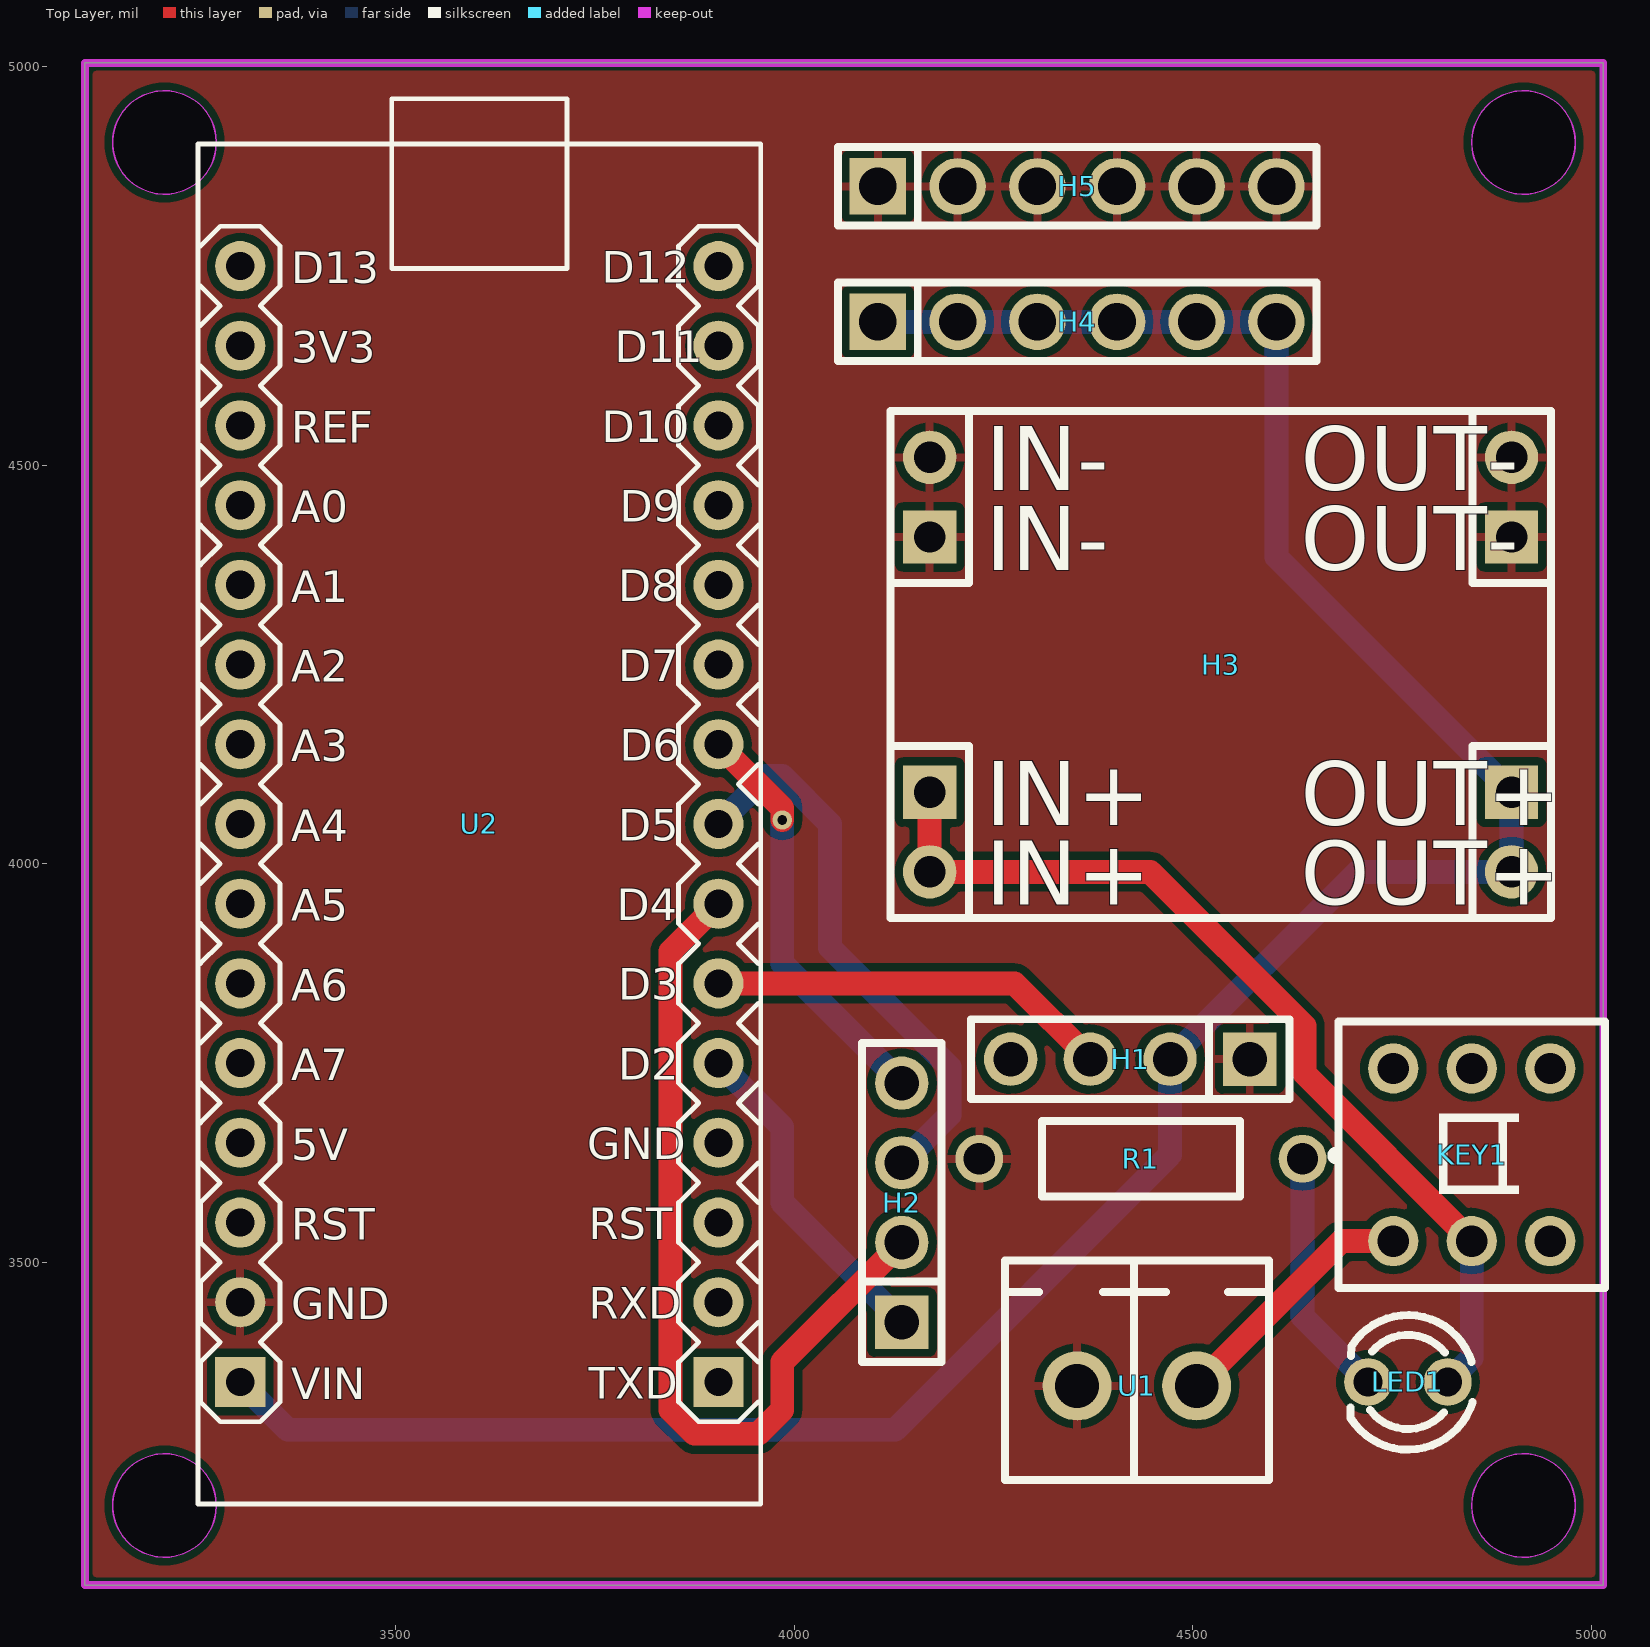
[diagram p0: Top Layer view]
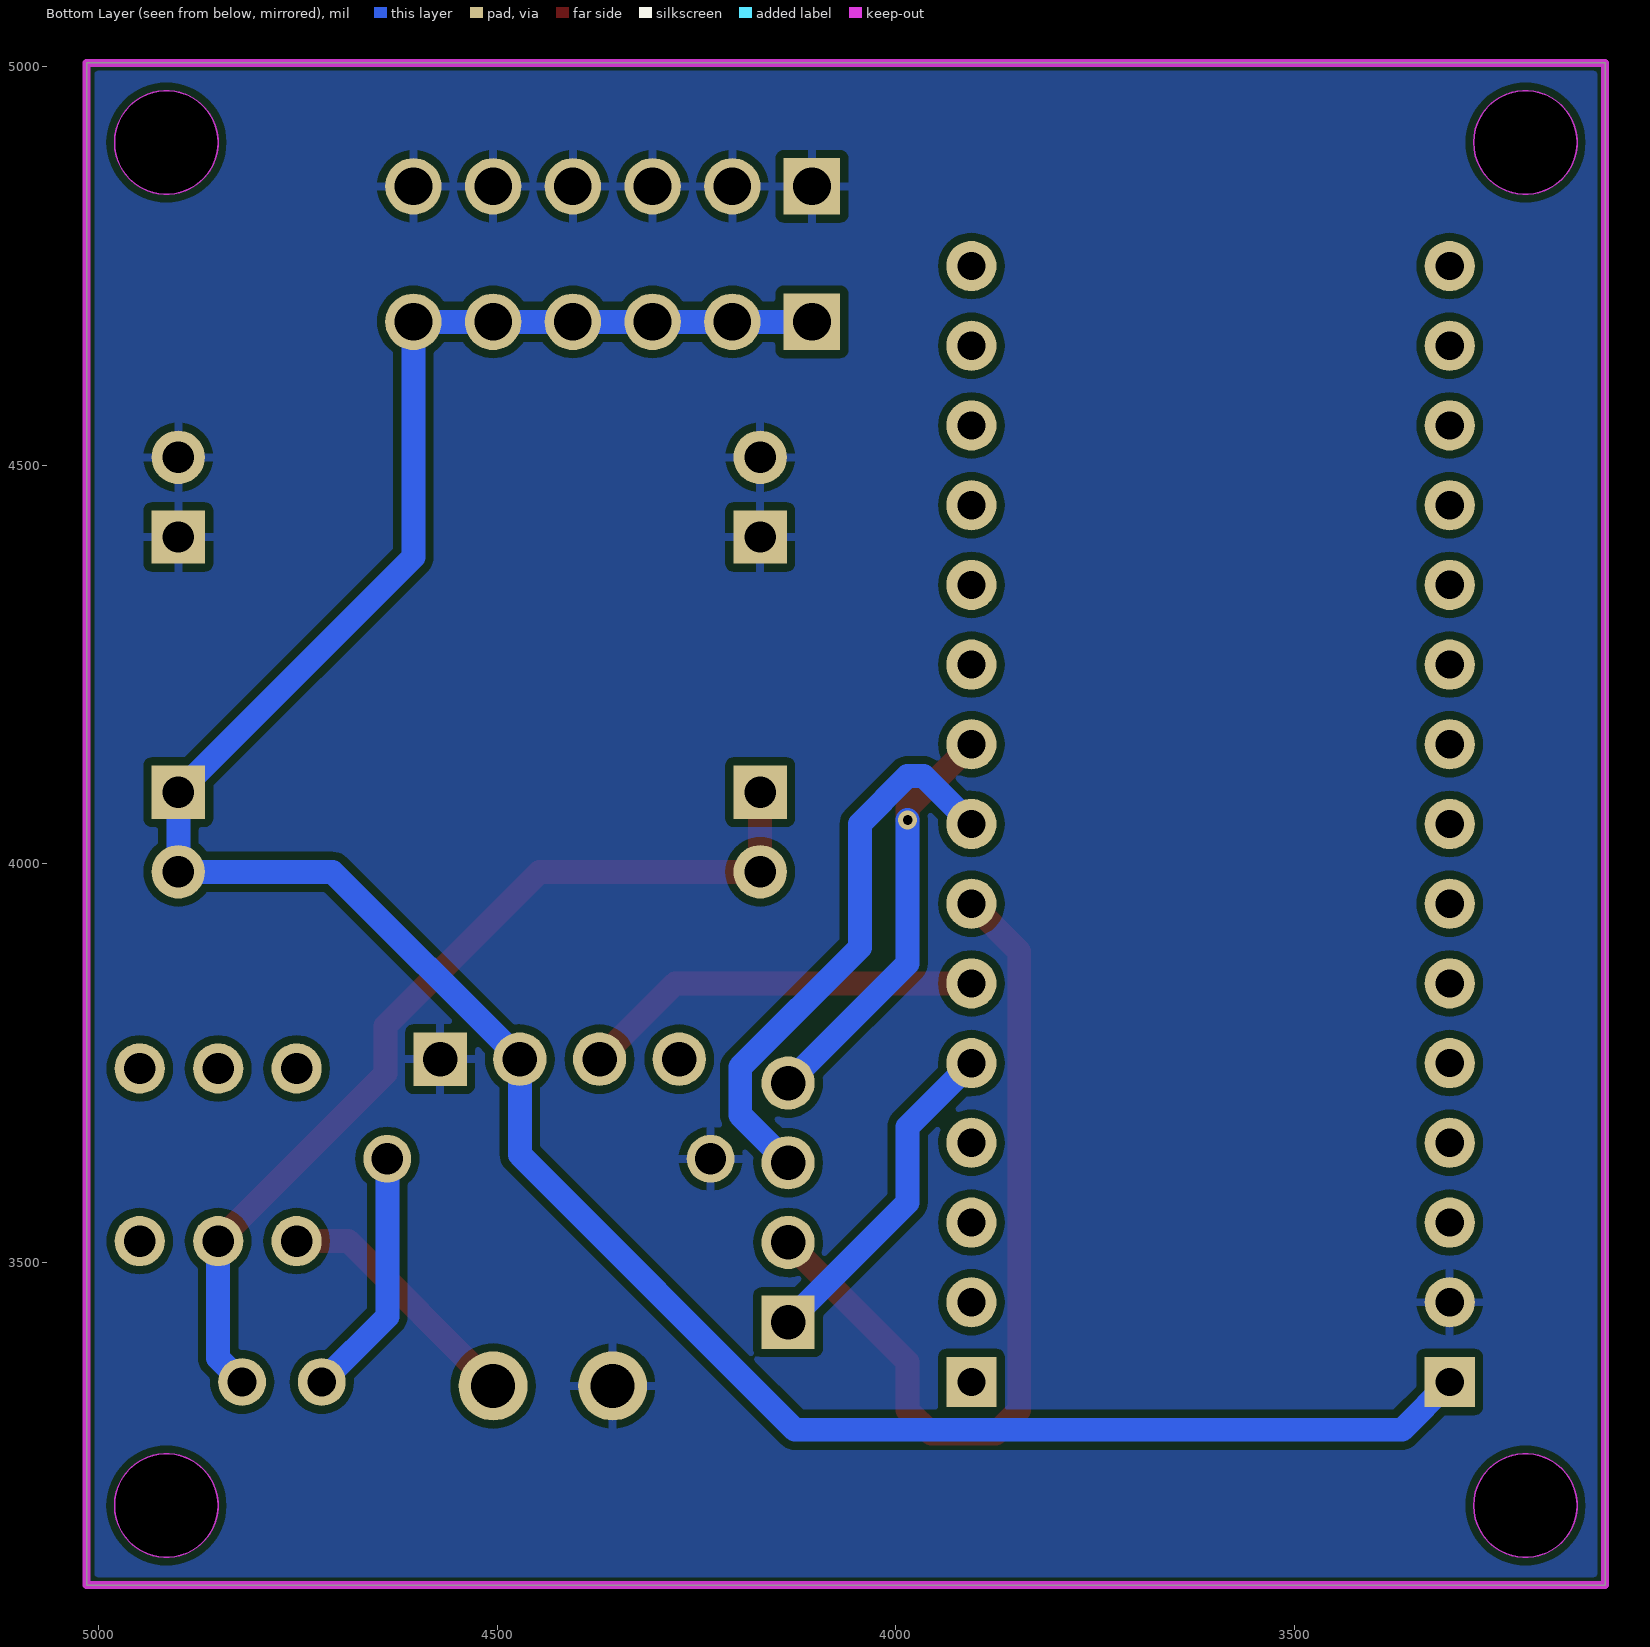
[diagram p1: Bottom Layer view, seen from below]
# Altium PCB MISC49855.pcbdoc
Units mil, origin at the board's own origin, x right, y up, seen from the top; angles counter-clockwise.
Board outline 1905 x 1910 mil, 2 copper layers (Top Layer, Bottom Layer), stack 62.206 mil thick; 10 components, 10 nets, 70 pads, 1 vias.

## Layer stack, top to bottom
Top Solder Mask Layer: solder mask 0.394, Dk 3.3
Top Layer: signal copper 1.379
Dielectric1: surface 59.449, FR4, Dk 4.5
Bottom Layer: signal copper 1.378
Bottom Solder Mask Layer: solder mask 0.394, Dk 3.3

## Board outline
3110,5005 3110,3095 5015,3095 5015,5005
cut-out: 3275,3195 cw(c3210,3195) 3145,3195 cw(c3210,3195)
cut-out: 4980,3195 cw(c4915,3195) 4850,3195 cw(c4915,3195)
cut-out: 4980,4905 cw(c4915,4905) 4850,4905 cw(c4915,4905)
cut-out: 3275,4905 cw(c3210,4905) 3145,4905 cw(c3210,4905)

## Design rules (kind name [scope] priority, off if disabled: settings)
BoardOutlineClearance copperThickness2oz_1 [All] p2 off: genericclearance=7.99 ignorepadtopadclearanceinfootprint=FALSE except(0: Arc-SplitContinuation Track-SplitContinuation SMDPad-SplitContinuation THPad-SplitContinuation Via-SplitContinuation Fill-SplitContinuation Region-SplitContinuation Poly-SplitContinuation Text-SplitContinuation Hole-SplitContinuation; 5.98: Arc-CutoutEdge Track-CutoutEdge SMDPad-CutoutEdge THPad-CutoutEdge Via-CutoutEdge Text-CutoutEdge; 6.89: Hole-OutlineEdge Hole-CutoutEdge; 10: Poly-OutlineEdge Poly-CutoutEdge; 11.81: Arc-OutlineEdge Track-OutlineEdge SMDPad-OutlineEdge THPad-OutlineEdge Via-OutlineEdge Fill-OutlineEdge Region-OutlineEdge Text-OutlineEdge Fill-CutoutEdge Region-CutoutEdge)
BoardOutlineClearance Plane_innerPlane_1 [All] p4 off: genericclearance=4.02 ignorepadtopadclearanceinfootprint=FALSE except(0: Arc-SplitContinuation Track-SplitContinuation SMDPad-SplitContinuation THPad-SplitContinuation Via-SplitContinuation Fill-SplitContinuation Region-SplitContinuation Poly-SplitContinuation Text-SplitContinuation Hole-SplitContinuation; 5.98: Arc-CutoutEdge Track-CutoutEdge SMDPad-CutoutEdge THPad-CutoutEdge Via-CutoutEdge Text-CutoutEdge; 6.89: Hole-OutlineEdge Hole-CutoutEdge; 10: Poly-OutlineEdge Poly-CutoutEdge; 11.81: Arc-OutlineEdge Track-OutlineEdge SMDPad-OutlineEdge THPad-OutlineEdge Via-OutlineEdge Fill-OutlineEdge Region-OutlineEdge Text-OutlineEdge Fill-CutoutEdge Region-CutoutEdge)
BoardOutlineClearance Copper_copperRegion_1 [All] p6 off: genericclearance=4.02 ignorepadtopadclearanceinfootprint=FALSE except(0: Arc-SplitContinuation Track-SplitContinuation SMDPad-SplitContinuation THPad-SplitContinuation Via-SplitContinuation Fill-SplitContinuation Region-SplitContinuation Poly-SplitContinuation Text-SplitContinuation Hole-SplitContinuation; 5.98: Arc-CutoutEdge Track-CutoutEdge SMDPad-CutoutEdge THPad-CutoutEdge Via-CutoutEdge Text-CutoutEdge; 6.89: Hole-OutlineEdge Hole-CutoutEdge; 10: Poly-OutlineEdge Poly-CutoutEdge; 11.81: Arc-OutlineEdge Track-OutlineEdge SMDPad-OutlineEdge THPad-OutlineEdge Via-OutlineEdge Fill-OutlineEdge Region-OutlineEdge Text-OutlineEdge Fill-CutoutEdge Region-CutoutEdge)
BoardOutlineClearance copperThickness1oz_1 [All] p8: genericclearance=4.02 ignorepadtopadclearanceinfootprint=FALSE except(0: Arc-SplitContinuation Track-SplitContinuation SMDPad-SplitContinuation THPad-SplitContinuation Via-SplitContinuation Fill-SplitContinuation Region-SplitContinuation Poly-SplitContinuation Text-SplitContinuation Hole-SplitContinuation; 5.98: Arc-CutoutEdge Track-CutoutEdge SMDPad-CutoutEdge THPad-CutoutEdge Via-CutoutEdge Text-CutoutEdge; 6.89: Hole-OutlineEdge Hole-CutoutEdge; 10: Poly-OutlineEdge Poly-CutoutEdge; 11.81: Arc-OutlineEdge Track-OutlineEdge SMDPad-OutlineEdge THPad-OutlineEdge Via-OutlineEdge Fill-OutlineEdge Region-OutlineEdge Text-OutlineEdge Fill-CutoutEdge Region-CutoutEdge)
Clearance copperThickness2oz [All] p1 off: gap=7.99 ignorepadtopadclearanceinfootprint=FALSE except(5.98: SMDPad-Track SMDPad-SMDPad THPad-Track SMDPad-THPad THPad-THPad Track-Via SMDPad-Via THPad-Via Via-Via Fill-SMDPad Region-SMDPad Fill-THPad Region-THPad Fill-Via Region-Via Fill-Fill Fill-Region Region-Region Arc-Track Arc-SMDPad Arc-THPad Arc-Via Fill-Arc Region-Arc Arc-Arc Text-Track SMDPad-Text Text-THPad Text-Via Fill-Text Region-Text Arc-Text Text-Text; 6.89: Hole-Track Hole-SMDPad Hole-THPad Hole-Via Fill-Hole Region-Hole Hole-Arc Hole-Text; 10: Poly-Track Poly-SMDPad Poly-THPad Poly-Via Poly-Fill Poly-Region Poly-Poly Poly-Arc Poly-Text Poly-Hole; 11.81: Fill-Track Region-Track)
Clearance Plane_innerPlane [All] p3 off: gap=4.02 ignorepadtopadclearanceinfootprint=FALSE except(5.98: SMDPad-Track SMDPad-SMDPad THPad-Track SMDPad-THPad THPad-THPad Track-Via SMDPad-Via THPad-Via Via-Via Fill-SMDPad Region-SMDPad Fill-THPad Region-THPad Fill-Via Region-Via Fill-Fill Fill-Region Region-Region Arc-Track Arc-SMDPad Arc-THPad Arc-Via Fill-Arc Region-Arc Arc-Arc Text-Track SMDPad-Text Text-THPad Text-Via Fill-Text Region-Text Arc-Text Text-Text; 6.89: Hole-Track Hole-SMDPad Hole-THPad Hole-Via Fill-Hole Region-Hole Hole-Arc Hole-Text; 10: Poly-Track Poly-SMDPad Poly-THPad Poly-Via Poly-Fill Poly-Region Poly-Poly Poly-Arc Poly-Text Poly-Hole; 11.81: Fill-Track Region-Track)
Clearance Copper_copperRegion [All] p5 off: gap=4.02 ignorepadtopadclearanceinfootprint=FALSE except(5.98: SMDPad-Track SMDPad-SMDPad THPad-Track SMDPad-THPad THPad-THPad Track-Via SMDPad-Via THPad-Via Via-Via Fill-SMDPad Region-SMDPad Fill-THPad Region-THPad Fill-Via Region-Via Fill-Fill Fill-Region Region-Region Arc-Track Arc-SMDPad Arc-THPad Arc-Via Fill-Arc Region-Arc Arc-Arc Text-Track SMDPad-Text Text-THPad Text-Via Fill-Text Region-Text Arc-Text Text-Text; 6.89: Hole-Track Hole-SMDPad Hole-THPad Hole-Via Fill-Hole Region-Hole Hole-Arc Hole-Text; 10: Poly-Track Poly-SMDPad Poly-THPad Poly-Via Poly-Fill Poly-Region Poly-Poly Poly-Arc Poly-Text Poly-Hole; 11.81: Fill-Track Region-Track)
Clearance copperThickness1oz [All] p7: gap=4.02 ignorepadtopadclearanceinfootprint=FALSE except(5.98: SMDPad-Track SMDPad-SMDPad THPad-Track SMDPad-THPad THPad-THPad Track-Via SMDPad-Via THPad-Via Via-Via Fill-SMDPad Region-SMDPad Fill-THPad Region-THPad Fill-Via Region-Via Fill-Fill Fill-Region Region-Region Arc-Track Arc-SMDPad Arc-THPad Arc-Via Fill-Arc Region-Arc Arc-Arc Text-Track SMDPad-Text Text-THPad Text-Via Fill-Text Region-Text Arc-Text Text-Text; 6.89: Hole-Track Hole-SMDPad Hole-THPad Hole-Via Fill-Hole Region-Hole Hole-Arc Hole-Text; 10: Poly-Track Poly-SMDPad Poly-THPad Poly-Via Poly-Fill Poly-Region Poly-Poly Poly-Arc Poly-Text Poly-Hole; 11.81: Fill-Track Region-Track)
DiffPairsRouting differentialPair [All] p1: maxlimit=6 minlimit=6 mostfreqgap=6 toplayer_minwidth=5 toplayer_prefwidth=10 toplayer_maxwidth=100 toplayer_mingap=6 toplayer_prefgap=6 toplayer_maxgap=6 bottomlayer_minwidth=5 bottomlayer_prefwidth=10 bottomlayer_maxwidth=100 bottomlayer_mingap=6 bottomlayer_prefgap=6 bottomlayer_maxgap=6 maxuncoupledlength=10
HoleToHoleClearance otherClearance [All] p1: gap=11.81 allowstackedmicrovias=TRUE
Length netLength [All] p1: minlimit=0 maxlimit=0
PasteMaskExpansion pasteMaskExpansion [All] p1: expansion=0
PlaneConnect innerPlane [All] p1: planeconnectstyle=Relief reliefexpansion=20 reliefentries=4 reliefconductorwidth=10 reliefairgap=10
PolygonConnect copperRegion [All] p1: connectstyle=Relief reliefconductorwidth=10 reliefentries=4 polygonreliefangle="90 Angle" airgapwidth=10 via.connectstyle=Relief via.reliefconductorwidth=10 via.reliefentries=4 via.polygonreliefangle="90 Angle" via.airgapwidth=10
RoutingVias viaSize [All] p1: holewidth=12.01 width=24.02 viastyle="Through Hole" minholewidth=11.81 minwidth=19.68 maxholewidth=248.03 maxwidth=393.7
SolderMaskExpansion solderMaskExpansion [IsVia] p1: expansion=-1000 istentingtop=TRUE
SolderMaskExpansion solderMaskExpansion [All] p2: expansion=2.01 istentingtop=FALSE
Width copperThickness2oz_2 [All] p1 off: maxlimit=100 minlimit=8 preferedwidth=10
Width copperThickness1oz_2 [All] p2: maxlimit=100 minlimit=5 preferedwidth=30

## Components (designator, comment, footprint, x,y, rotation, side; value= is the part's Value field where it differs from the comment)
H1 "" HDR-TH_4P-P2.54-V-M 4421.54,3755.05 r180 top
H2 "" HDR-TH_4P-P2.54-V-M 4135,3575 r90 top
H3 "" HDR-TH_8P-P2.54-V-M 4170,4510 r0 top
H4 "" HDR-TH_6P-P2.54-V-M-1 4355,4680 r0 top
H5 "" HDR-TH_6P-P2.54-V-M-1 4355,4850 r0 top
KEY1 "Self-locking switch" SW-TH_6P-L8.5-W8.5-P2.54 4850,3635 r0 top
LED1 "" LED_TH-3mm 4770,3350 r180 top
R1 "1kΩ" Res_1/4W 4435,3630 r180 top
U1 "2P-P3.81_KF2EDGV-3.81-2P" CONN-TH_2P-P3.81_KF2EDGV-3.81-2P 4430,3345 r180 top
U2 "ARDUINO_NANO" COMM-TH_ARDUINO_NANO 3605,4050 r270 top

## Footprints (in the part's own frame and the unit in brackets; to place one, negate y for a bottom-side part, rotate by r counter-clockwise, add the part's x,y. Pads: shape width x height; smd on the part's side, far side on the other; paste and mask are expansions set on the pad)
COMM-TH_ARDUINO_NANO [mm]
  rect 1.6x1.6 hole 0.9: 1(17.78,7.62) 30(17.78,-7.62)
  round 1.6 hole 0.9: 2(15.24,7.62) 4(10.16,7.62) 6(5.08,7.62) 8(0,7.62) 10(-5.08,7.62) 12(-10.16,7.62) 14(-15.24,7.62) 15(-17.78,7.62) 16(-17.78,-7.62) 18(-12.7,-7.62) 20(-7.62,-7.62) 22(-2.54,-7.62) 24(2.54,-7.62) 26(7.62,-7.62) 28(12.7,-7.62) 29(15.24,-7.62)
  round 1.6 hole 0.9 copper offset 0,0: 3(12.7,7.62)
  round 1.6 hole 0.9 copper offset -0.001,0: 5(7.621,7.62) 7(2.541,7.62) 9(-2.539,7.62) 11(-7.619,7.62) 13(-12.699,7.62)
  round 1.6 hole 0.9 copper offset 0.001,0: 17(-15.241,-7.62) 19(-10.161,-7.62) 21(-5.081,-7.62) 23(-0.001,-7.62) 25(5.079,-7.62) 27(10.159,-7.62)
  silkscreen extent -23.11,-8.97 21.67,8.97
CONN-TH_2P-P3.81_KF2EDGV-3.81-2P [mm]
  round 2.2 hole 1.4: 1(-1.905,0) 2(1.905,0)
  silkscreen extent -4.21,-4 4.21,3
HDR-TH_4P-P2.54-V-M [mm]
  rect 1.7x1.7 hole 1.1: 1(-3.81,0)
  round 1.7 hole 1.1: 2(-1.27,0) 3(1.27,0) 4(3.81,0)
  silkscreen extent -5.08,-1.27 5.08,1.27
HDR-TH_6P-P2.54-V-M-1 [mm]
  rect 1.8x1.8 hole 1.2: 1(-6.35,0)
  round 1.8 hole 1.2: 2(-3.81,0) 3(-1.27,0) 4(1.27,0) 5(3.81,0) 6(6.35,0)
  silkscreen extent -7.62,-1.25 7.62,1.25
HDR-TH_8P-P2.54-V-M [mm]
  round 1.7 hole 1: 1(0,0) 4(0,-13.208) 5(18.542,0) 8(18.542,-13.208)
  rect 1.7x1.7 hole 1: 2(0,-2.54) 3(0,-10.668) 6(18.542,-2.54) 7(18.542,-10.668)
  silkscreen extent -1.25,-14.68 19.79,1.47
LED_TH-3mm [mil]
  round 60 hole 36 paste+0 mask+2: 1(-50,0) 2(50,0)
  silkscreen extent -81,-84 72,85
Res_1/4W [mil]
  round 60 hole 39.37 paste+0 mask+2: 1(-202.76,0) 2(202.76,0)
  silkscreen extent -124,-47 124,47
SW-TH_6P-L8.5-W8.5-P2.54 [mm]
  round 1.6 hole 1: 1(-2.5,-2.75) 2(0,-2.75) 3(2.5,-2.75) 4(-2.5,2.75) 5(0,2.75) 6(2.5,2.75)
  silkscreen extent -4.47,-4.25 4.25,4.25

## Via types
v1: diameter 24.02, hole 12, Top Layer to Bottom Layer, 1 vias

## Nets (pads, with @x,y where several pads share a name; then routed paths per layer and width w, separated by ;. In a path a pad name is that pad's centre, name@x,y a point inside that pad or via, vN(x,y) a via of type N, cw(c..) or ccw(c..) an arc to the next point about the centre after c; other vN are vias at no path point)
5V: H1.2 H3.7 H3.8 H4.1 H4.2 H4.3 H4.4 H4.5 H4.6 U2.30 | length 3292.3
  Bottom Layer w30: U2.30 3365,3290 4126.49,3290 4471.54,3635.05 H1.2 4706.49,3990 H3.8 H3.7 4605,4385 H4.6 H4.5 H4.4 H4.3 H4.2 H4.1
12V: H3.3 H3.4 KEY1.2 LED1.1 | length 1196.2
  Top Layer w30: H3.3 H3.4 4446.73,3990 4639.99,3796.73 4639.99,3736.73 KEY1.2
  Bottom Layer w30: LED1.1 4849.99,3379.99 KEY1.2
$1N203: LED1.2 R1.1 | length 314.1
  Bottom Layer w30: R1.1 4637.76,3432.24 LED1.2
$1N384: KEY1.1 U1.1 | length 321.8
  Top Layer w30: U1.1 4686.73,3526.73 KEY1.1
ECHO: H2.4 U2.9 | length 520.3
  Top Layer w30: U2.9 3985,4070 v1(3985,4055)
  Bottom Layer w30: v1(3985,4055) 3985,3875 H2.4
GND: H1.1 H3.1 H3.2 H3.5 H3.6 H5.1 H5.2 H5.3 H5.4 H5.5 H5.6 R1.2 U1.2 U2.29
IN1: H2.1 U2.5 | length 420.3
  Bottom Layer w30: U2.5 3985,3670 3985,3575 H2.1
IN2: H2.2 U2.7 | length 1096.8
  Top Layer w30: U2.7 3845,3890 3845,3315 3875,3285 3955,3285 3985,3315 3985,3375 H2.2
SERVO: H1.3 U2.6 | length 505.9
  Top Layer w30: U2.6 4276.58,3850 H1.3
TRIG: H2.3 U2.8 | length 701.7
  Bottom Layer w30: U2.8 3965,4110 3985,4110 4045,4050 4045,3895 4195,3745 4195,3685 H2.3
pads on no net: H1.4 KEY1.3 KEY1.4 KEY1.5 KEY1.6 U2.1 U2.2 U2.3 U2.4 U2.10 U2.11 U2.12 U2.13 U2.14 U2.15 U2.16 U2.17 U2.18 U2.19 U2.20 U2.21 U2.22 U2.23 U2.24 U2.25 U2.26 U2.27 U2.28

## Polygon pours and split planes (outlines as drawn)
GND on Top Layer (solid, remove dead copper, pour order 0): 3000,5155 3000,3010 5125,3010 5125,5155
GND on Bottom Layer (solid, remove dead copper, pour order 2): 3055,5075 3055,3000 5100,3000 5100,5075

## Keep-outs
Board Outline Layer:
  region: 3275,3195 cw(c3210,3195) 3145,3195 cw(c3210,3195)
  circle w0.1: c3210,3195 r65
  region: 3275,3195 3274.62,3187.97 3273.48,3181.03 3271.6,3174.25 3268.99,3167.71 3265.7,3161.49 3261.75,3155.66 3257.19,3150.3 3252.08,3145.46 3246.48,3141.2 3240.45,3137.57 3234.06,3134.62 3227.39,3132.37 3220.52,3130.86 3213.52,3130.1 3206.48,3130.1 3199.48,3130.86 3192.61,3132.37 3185.94,3134.62 3179.55,3137.57 3173.52,3141.2 3167.92,3145.46 3162.81,3150.3 3158.25,3155.66 3154.3,3161.49 3151.01,3167.71 3148.4,3174.25 3146.52,3181.03 3145.38,3187.97 3145,3195 3145.38,3202.03 3146.52,3208.97 3148.4,3215.75 3151.01,3222.29 3154.3,3228.51 3158.25,3234.34 3162.81,3239.7 3167.92,3244.54 3173.52,3248.8 3179.55,3252.43 3185.94,3255.38 3192.61,3257.63 3199.48,3259.14 3206.48,3259.9 3213.52,3259.9 3220.52,3259.14 3227.39,3257.63 3234.06,3255.38 3240.45,3252.43 3246.48,3248.8 3252.08,3244.54 3257.19,3239.7 3261.75,3234.34 3265.7,3228.51 3268.99,3222.29 3271.6,3215.75 3273.48,3208.97 3274.62,3202.03
  region: 4980,3195 cw(c4915,3195) 4850,3195 cw(c4915,3195)
  circle w0.1: c4915,3195 r65
  region: 4980,3195 4979.62,3187.97 4978.48,3181.03 4976.6,3174.25 4973.99,3167.71 4970.7,3161.49 4966.75,3155.66 4962.19,3150.3 4957.08,3145.46 4951.48,3141.2 4945.45,3137.57 4939.06,3134.62 4932.39,3132.37 4925.52,3130.86 4918.52,3130.1 4911.48,3130.1 4904.48,3130.86 4897.61,3132.37 4890.94,3134.62 4884.55,3137.57 4878.52,3141.2 4872.92,3145.46 4867.81,3150.3 4863.25,3155.66 4859.3,3161.49 4856.01,3167.71 4853.4,3174.25 4851.52,3181.03 4850.38,3187.97 4850,3195 4850.38,3202.03 4851.52,3208.97 4853.4,3215.75 4856.01,3222.29 4859.3,3228.51 4863.25,3234.34 4867.81,3239.7 4872.92,3244.54 4878.52,3248.8 4884.55,3252.43 4890.94,3255.38 4897.61,3257.63 4904.48,3259.14 4911.48,3259.9 4918.52,3259.9 4925.52,3259.14 4932.39,3257.63 4939.06,3255.38 4945.45,3252.43 4951.48,3248.8 4957.08,3244.54 4962.19,3239.7 4966.75,3234.34 4970.7,3228.51 4973.99,3222.29 4976.6,3215.75 4978.48,3208.97 4979.62,3202.03
  region: 4980,4905 cw(c4915,4905) 4850,4905 cw(c4915,4905)
  circle w0.1: c4915,4905 r65
  region: 4980,4905 4979.62,4897.97 4978.48,4891.03 4976.6,4884.25 4973.99,4877.71 4970.7,4871.49 4966.75,4865.66 4962.19,4860.3 4957.08,4855.46 4951.48,4851.2 4945.45,4847.57 4939.06,4844.62 4932.39,4842.37 4925.52,4840.86 4918.52,4840.1 4911.48,4840.1 4904.48,4840.86 4897.61,4842.37 4890.94,4844.62 4884.55,4847.57 4878.52,4851.2 4872.92,4855.46 4867.81,4860.3 4863.25,4865.66 4859.3,4871.49 4856.01,4877.71 4853.4,4884.25 4851.52,4891.03 4850.38,4897.97 4850,4905 4850.38,4912.03 4851.52,4918.97 4853.4,4925.75 4856.01,4932.29 4859.3,4938.51 4863.25,4944.34 4867.81,4949.7 4872.92,4954.54 4878.52,4958.8 4884.55,4962.43 4890.94,4965.38 4897.61,4967.63 4904.48,4969.14 4911.48,4969.9 4918.52,4969.9 4925.52,4969.14 4932.39,4967.63 4939.06,4965.38 4945.45,4962.43 4951.48,4958.8 4957.08,4954.54 4962.19,4949.7 4966.75,4944.34 4970.7,4938.51 4973.99,4932.29 4976.6,4925.75 4978.48,4918.97 4979.62,4912.03
  region: 3275,4905 cw(c3210,4905) 3145,4905 cw(c3210,4905)
  circle w0.1: c3210,4905 r65
  region: 3275,4905 3274.62,4897.97 3273.48,4891.03 3271.6,4884.25 3268.99,4877.71 3265.7,4871.49 3261.75,4865.66 3257.19,4860.3 3252.08,4855.46 3246.48,4851.2 3240.45,4847.57 3234.06,4844.62 3227.39,4842.37 3220.52,4840.86 3213.52,4840.1 3206.48,4840.1 3199.48,4840.86 3192.61,4842.37 3185.94,4844.62 3179.55,4847.57 3173.52,4851.2 3167.92,4855.46 3162.81,4860.3 3158.25,4865.66 3154.3,4871.49 3151.01,4877.71 3148.4,4884.25 3146.52,4891.03 3145.38,4897.97 3145,4905 3145.38,4912.03 3146.52,4918.97 3148.4,4925.75 3151.01,4932.29 3154.3,4938.51 3158.25,4944.34 3162.81,4949.7 3167.92,4954.54 3173.52,4958.8 3179.55,4962.43 3185.94,4965.38 3192.61,4967.63 3199.48,4969.14 3206.48,4969.9 3213.52,4969.9 3220.52,4969.14 3227.39,4967.63 3234.06,4965.38 3240.45,4962.43 3246.48,4958.8 3252.08,4954.54 3257.19,4949.7 3261.75,4944.34 3265.7,4938.51 3268.99,4932.29 3271.6,4925.75 3273.48,4918.97 3274.62,4912.03
  lines w10: 3110,3095 3110,5005 5015,5005 5015,3095 3110,3095

## Silkscreen, mask and mechanical layers (free items; w line width, h text height)
Mechanical Layer:
  circle w0.1: c3210,3195 r65
  circle w0.1: c4915,3195 r65
  circle w0.1: c4915,4905 r65
  circle w0.1: c3210,4905 r65